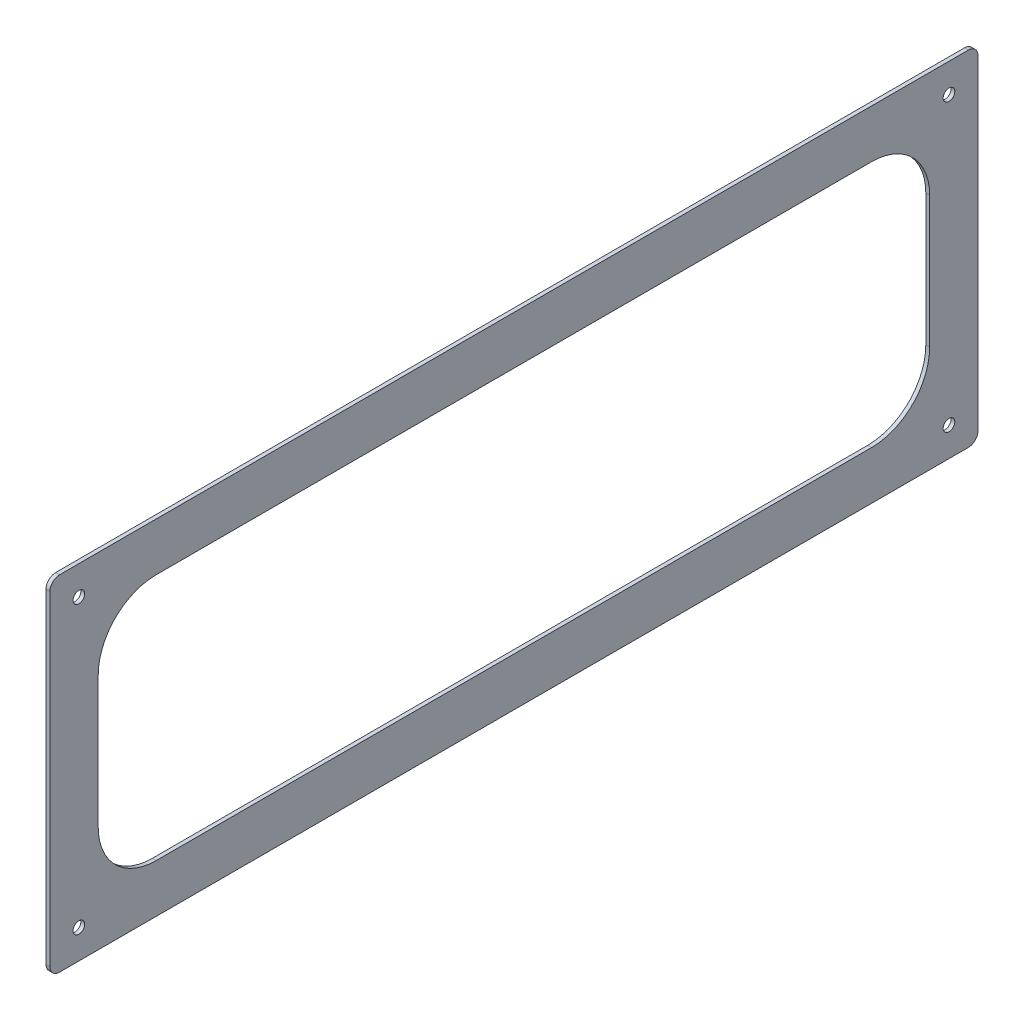
from build123d import *

# Parameters (mm, degrees)
SKETCH_1_W          = 480
SKETCH_1_H          = 178
EXTRUDE_1_DEPTH     = 2
SKETCH_2_R          = 3
CUT_EXTRUDE_1_DEPTH = 256.978514723
FILLET_1_R          = 5
SKETCH_3_W          = 430
SKETCH_3_H          = 128
CUT_EXTRUDE_2_DEPTH = 256.978514723
FILLET_2_R          = 30


with BuildPart() as part:
    # 草图1 → 凸台-拉伸1 (new body)
    with BuildSketch(Plane(origin=(0, 0, 0), x_dir=(0, 0, -1), z_dir=(1, 0, 0))):
        Rectangle(SKETCH_1_W, SKETCH_1_H)
    extrude(amount=EXTRUDE_1_DEPTH)

    # 草图2 → 切除-拉伸1 (cut, through all)
    with BuildSketch(Plane(origin=(2, 0, 0), x_dir=(0, 0, -1), z_dir=(1, 0, 0))):
        with Locations((-225, 74)):
            Circle(SKETCH_2_R)
        with Locations((225, 74)):
            Circle(SKETCH_2_R)
        with Locations((-225, -74)):
            Circle(SKETCH_2_R)
        with Locations((225, -74)):
            Circle(SKETCH_2_R)
    extrude(amount=-CUT_EXTRUDE_1_DEPTH, mode=Mode.SUBTRACT)

    # 圆角1
    fillet_1_edges = [part.edges().sort_by_distance(p)[0] for p in [
        (1, 89, 240),
        (1, 89, -240),
        (1, -89, -240),
        (1, -89, 240),
    ]]
    fillet(fillet_1_edges, radius=FILLET_1_R)

    # 草图3 → 切除-拉伸2 (cut, through all)
    with BuildSketch(Plane(origin=(2, 0, 0), x_dir=(0, 0, -1), z_dir=(1, 0, 0))):
        Rectangle(SKETCH_3_W, SKETCH_3_H)
    extrude(amount=-CUT_EXTRUDE_2_DEPTH, mode=Mode.SUBTRACT)

    # 圆角2
    fillet_2_edges = [part.edges().sort_by_distance(p)[0] for p in [
        (1, -64, 215),
        (1, 64, 215),
        (1, 64, -215),
        (1, -64, -215),
    ]]
    fillet(fillet_2_edges, radius=FILLET_2_R)


solid = part.part
